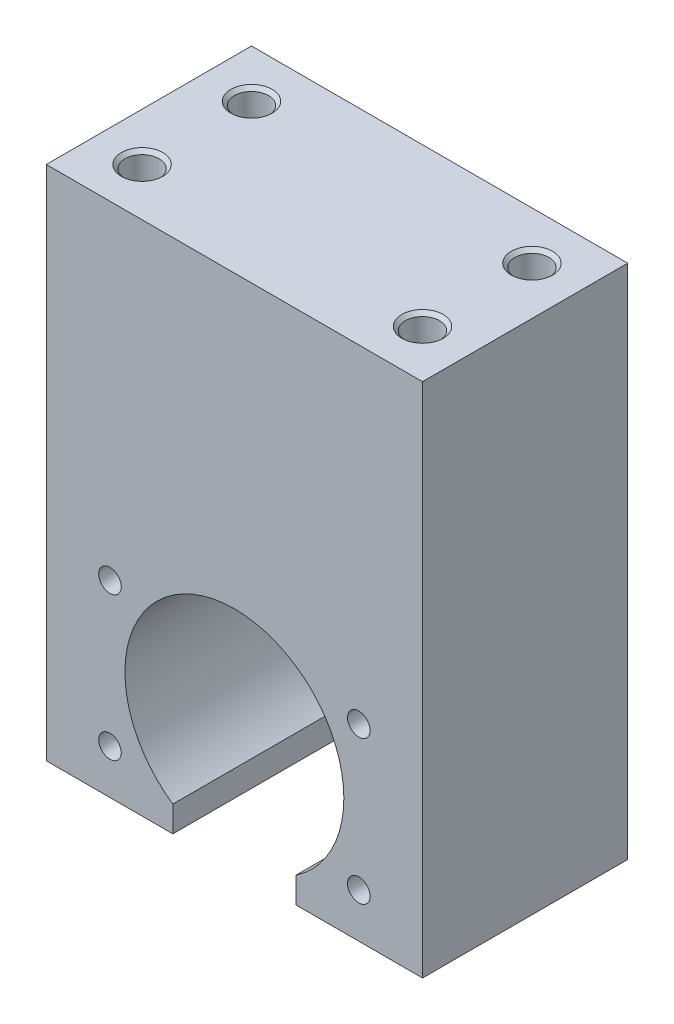
SolidWorks part; units mm, degrees
ref_plane "前视基准面" through (0, 0, 0) normal (0, 0, 1) x (1, 0, 0)
ref_plane "上视基准面" through (0, 0, 0) normal (0, 1, 0) x (1, 0, 0)
ref_plane "右视基准面" through (0, 0, 0) normal (1, 0, 0) x (0, 0, -1)
sketch "草图1" plane through (0, 0, 0) normal (0, 0, 1) x (1, 0, 0)
  line L0 (-27.5, 58.5) -> (27.5, 58.5)
  line L1 (27.5, 58.5) -> (27.5, -17)
  line L2 (27.5, -17) -> (9, -17)
  line L3 (9, -17) -> (9, -13.2288)
  line L4 (-27.5, 58.5) -> (-27.5, -17)
  line L5 (-27.5, -17) -> (-9, -17)
  line L6 (-9, -17) -> (-9, -13.2288)
  arc A0 (9, -13.2288) -> (-9, -13.2288) centre (0, 0) ccw
extrude "凸台-拉伸1" add sketch "草图1" along normal mid plane 30
hole_wizard "M4 螺纹孔1" positions "草图3" profile "草图2" tap size "M4" standard "GB"
sketch "草图3" plane through (0, 0, 15) normal (0, 0, 1) x (1, 0, 0)
  circle A0 centre (18.1865, 10.5) radius 2.25 construction
  circle A1 centre (18.1865, -10.5) radius 2.25 construction
  circle A2 centre (-18.1865, -10.5) radius 2.25 construction
  circle A3 centre (-18.1865, 10.5) radius 2.25 construction
  point P1 (18.1865, 10.5)
  point P5 (18.1865, -10.5)
  point P9 (-18.1865, -10.5)
  point P13 (-18.1865, 10.5)
cosmetic thread "孔螺蚊线1" parameters "D1"=6, "D2"=4
cosmetic thread "孔螺蚊线2" parameters "D1"=6, "D2"=4
cosmetic thread "孔螺蚊线3" parameters "D1"=6, "D2"=4
cosmetic thread "孔螺蚊线4" parameters "D1"=6, "D2"=4
sketch "草图2" plane through (18.1865, 10.5, 15) normal (1, 0, 0) x (0, -1, 0)
  line L0 (0, 0) -> (0, 10.4914)
  line L1 (0, 10.4914) -> (1.65, 9.5)
  line L2 (1.65, 9.5) -> (1.65, 0)
  line L5 (1.65, 0) -> (0, 0)
  line L10 (0, 10.4914) -> (-1.65, 9.5) construction
  line L11 (0, -6.35) -> (0, 107.95) construction
  dimension "螺纹孔钻头直径" = 3.3
  dimension "螺纹孔钻头深度" = 9.5
  dimension "导头角度" = 118
sketch "草图4" plane through (0, 58.5, 0) normal (0, 1, 0) x (1, 0, 0)
  line L0 (27.5, -15) -> (27.5, 15) construction
  line L1 (-20.5, -8) -> (20.5, -8)
  line L2 (-20.5, -8) -> (-20.5, 8)
  line L3 (-20.5, 8) -> (20.5, 8)
  line L4 (20.5, -8) -> (20.5, 8)
  line L5 (-20.5, -8) -> (20.5, 8) construction
  line L6 (-20.5, 8) -> (20.5, -8) construction
  line L7 (27.5, -15) -> (-27.5, -15) construction
  point P0 (0, 0)
  dimension "D1" = 7
  dimension "D2" = 7
hole_wizard "M6 螺纹孔1" positions "3D草图1" profile "草图5" tap size "M6" standard "GB"
sketch3d "3D草图1"
  point P0 (-20.5, 58.5, 8)
  point P3 (-20.5, 58.5, -8)
  point P6 (20.5, 58.5, -8)
  point P9 (20.5, 58.5, 8)
sketch "草图5" plane through (-20.5, 58.5, 8) normal (1, 0, 0) x (0, 0, 1)
  line L0 (0, 0) -> (0, 13.5022)
  line L1 (0, 13.5022) -> (2.5, 12)
  line L2 (2.5, 12) -> (2.5, 0.525)
  line L3 (2.5, 0.525) -> (3.025, 0)
  line L5 (3.025, 0) -> (0, 0)
  line L6 (-2.5, 0.525) -> (-3.025, 0) construction
  line L10 (0, 13.5022) -> (-2.5, 12) construction
  line L11 (0, -6.35) -> (0, 107.95) construction
  dimension "螺纹孔钻头直径" = 5
  dimension "螺纹孔钻头深度" = 12
  dimension "近端锥形沉头孔直径" = 6.05
  dimension "近端锥形沉头孔角度" = 90
  dimension "导头角度" = 118
cosmetic thread "孔螺蚊线5" parameters "D1"=8, "D2"=6
cosmetic thread "孔螺蚊线6" parameters "D1"=8, "D2"=6
cosmetic thread "孔螺蚊线7" parameters "D1"=8, "D2"=6
cosmetic thread "孔螺蚊线8" parameters "D1"=8, "D2"=6
equation "\"D3@草图1\"=\"D2@草图1\""
